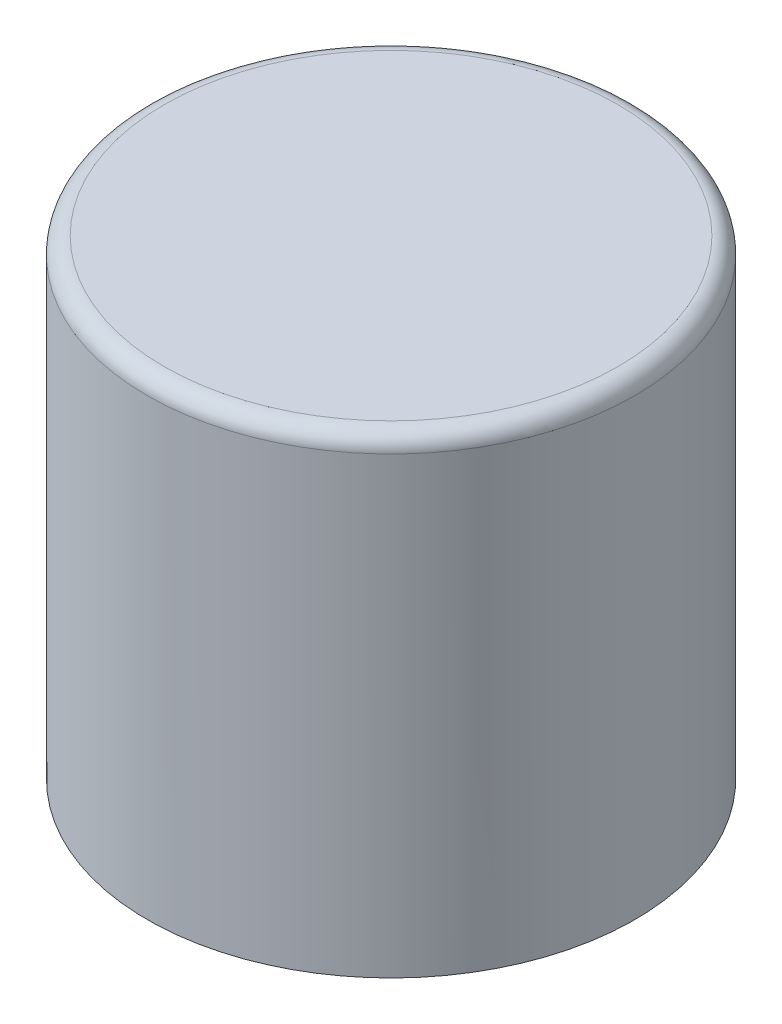
from build123d import *

# Parameters (mm, degrees)
SKETCH_1_W   = 2
SKETCH_1_H   = 26
SKETCH_1_H_2 = 2
SKETCH_1_W_2 = 12.5
FILLET_1_R   = 1


with BuildPart() as part:
    # 草图1 → 旋转1 (revolve)
    with BuildSketch(Plane.XY, mode=Mode.PRIVATE) as revolve_1_sk:
        with Locations((13.5, -15)):
            Rectangle(SKETCH_1_W, SKETCH_1_H)
        with Locations((13.5, -1)):
            Rectangle(SKETCH_1_W, SKETCH_1_H_2)
        with Locations((6.25, -1)):
            Rectangle(SKETCH_1_W_2, SKETCH_1_H_2)
    revolve(revolve_1_sk.sketch.rotate(Axis((0, -2, 0), (0, 1, 0)), 90), axis=Axis((0, -2, 0), (0, 1, 0)))

    # 圆角1
    fillet_1_edges = [part.edges().sort_by_distance(p)[0] for p in [
        (0, 0, 14.5),
    ]]
    fillet(fillet_1_edges, radius=FILLET_1_R)


solid = part.part
